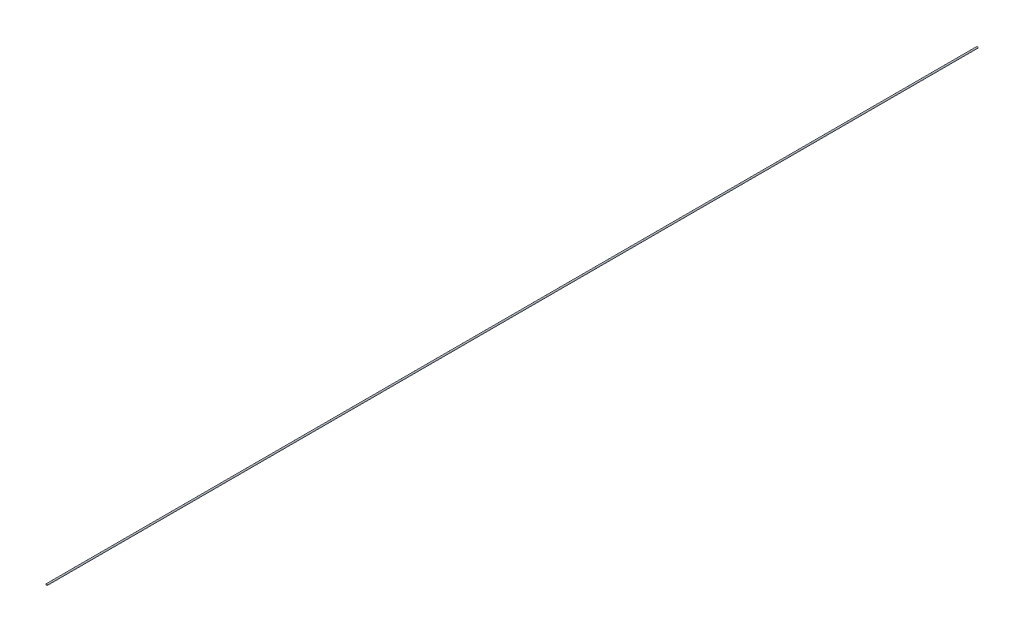
from build123d import *

# Parameters (mm, degrees)
SKETCH1_R           = 1.5
SKETCH1_R_2         = 0.15
BOSS_EXTRUDE1_DEPTH = 1900


with BuildPart() as part:
    # Sketch1 → Boss-Extrude1 (new body)
    with BuildSketch(Plane.XY):
        with Locations(Location((0, 0, 0), (0, 0, 180))):
            Circle(SKETCH1_R)
        with Locations((0, 0.95)):
            Circle(SKETCH1_R_2, mode=Mode.SUBTRACT)
        with Locations((0.822724134, -0.475)):
            Circle(SKETCH1_R_2, mode=Mode.SUBTRACT)
        with Locations((-0.822724134, -0.475)):
            Circle(SKETCH1_R_2, mode=Mode.SUBTRACT)
    extrude(amount=BOSS_EXTRUDE1_DEPTH)


solid = part.part
